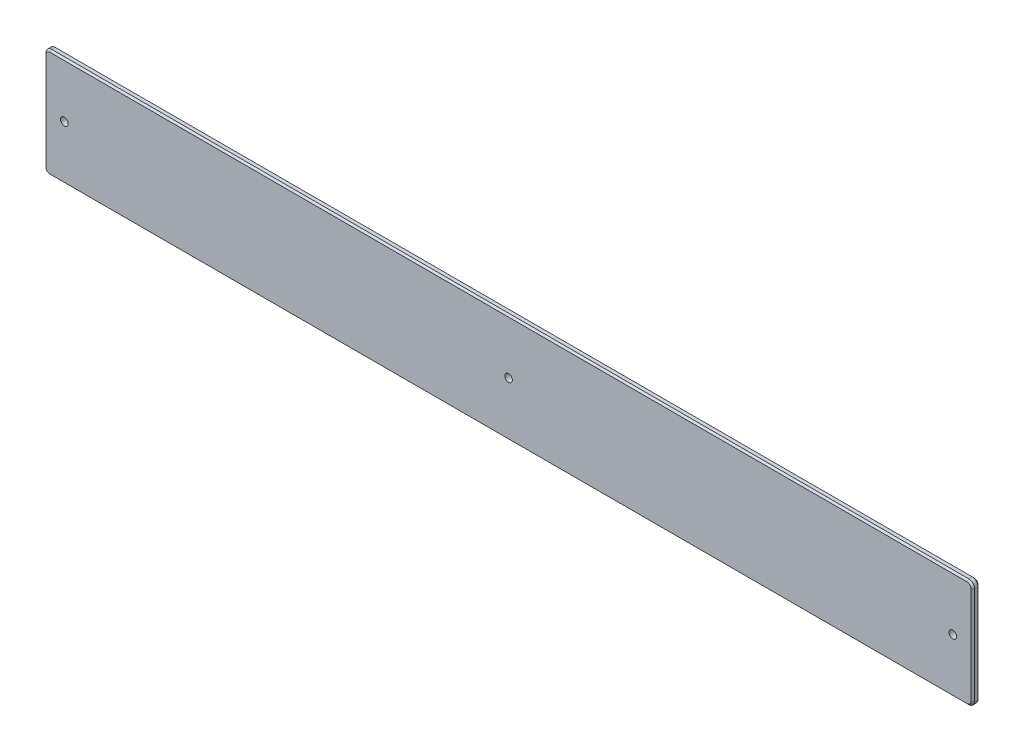
SolidWorks part; units mm, degrees
material "Aluminum Profile"
ref_plane "Front Plane" through (0, 0, 0) normal (0, 0, 1) x (1, 0, 0)
ref_plane "Top Plane" through (0, 0, 0) normal (0, 1, 0) x (1, 0, 0)
ref_plane "Right Plane" through (0, 0, 0) normal (1, 0, 0) x (0, 0, -1)
sketch "Sketch1" plane through (0, 0, 0) normal (0, 0, 1) x (1, 0, 0)
  line L1 (405, -47.5) -> (-405, -47.5)
  line L2 (405, -47.5) -> (405, 47.5)
  line L3 (405, 47.5) -> (-405, 47.5)
  line L4 (-405, -47.5) -> (-405, 47.5)
  line L5 (405, -47.5) -> (-405, 47.5) construction
  line L6 (405, 47.5) -> (-405, -47.5) construction
  point P0 (0, 0)
  dimension "D1" = 95
  dimension "D2" = 810
extrude "Boss-Extrude1" add sketch "Sketch1" along normal blind 6
fillet "Fillet1" radius 5 4 edges at (405, 47.5, 3) (405, -47.5, 3) (-405, -47.5, 3) (-405, 47.5, 3)
chamfer "Chamfer1" distance 1.5 angle 45 16 edges at (-403.5355, 46.0355, 0) (-405, 0, 0) (-403.5355, -46.0355, 0) (0, -47.5, 0) (403.5355, -46.0355, 0) (405, 0, 0) (403.5355, 46.0355, 0) (0, 47.5, 0) (403.5355, -46.0355, 6) (0, -47.5, 6) (-403.5355, -46.0355, 6) (-405, 0, 6) (-403.5355, 46.0355, 6) (0, 47.5, 6) (403.5355, 46.0355, 6) (405, 0, 6)
sketch "Sketch2" plane through (0, 0, 6) normal (0, 0, 1) x (1, 0, 0)
  line L0 (-387.5, 0) -> (0, 0) construction
  line L1 (0, 0) -> (387.5, 0) construction
  line L2 (-405, -42.5) -> (-405, 42.5) construction
  circle A0 centre (-387.5, 0) radius 3.3
  circle A1 centre (0, 0) radius 3.3
  circle A2 centre (387.5, 0) radius 3.3
  dimension "D2" = 6.6
  dimension "D1" = 17.5
extrude "Cut-Extrude1" cut sketch "Sketch2" against normal up to next
